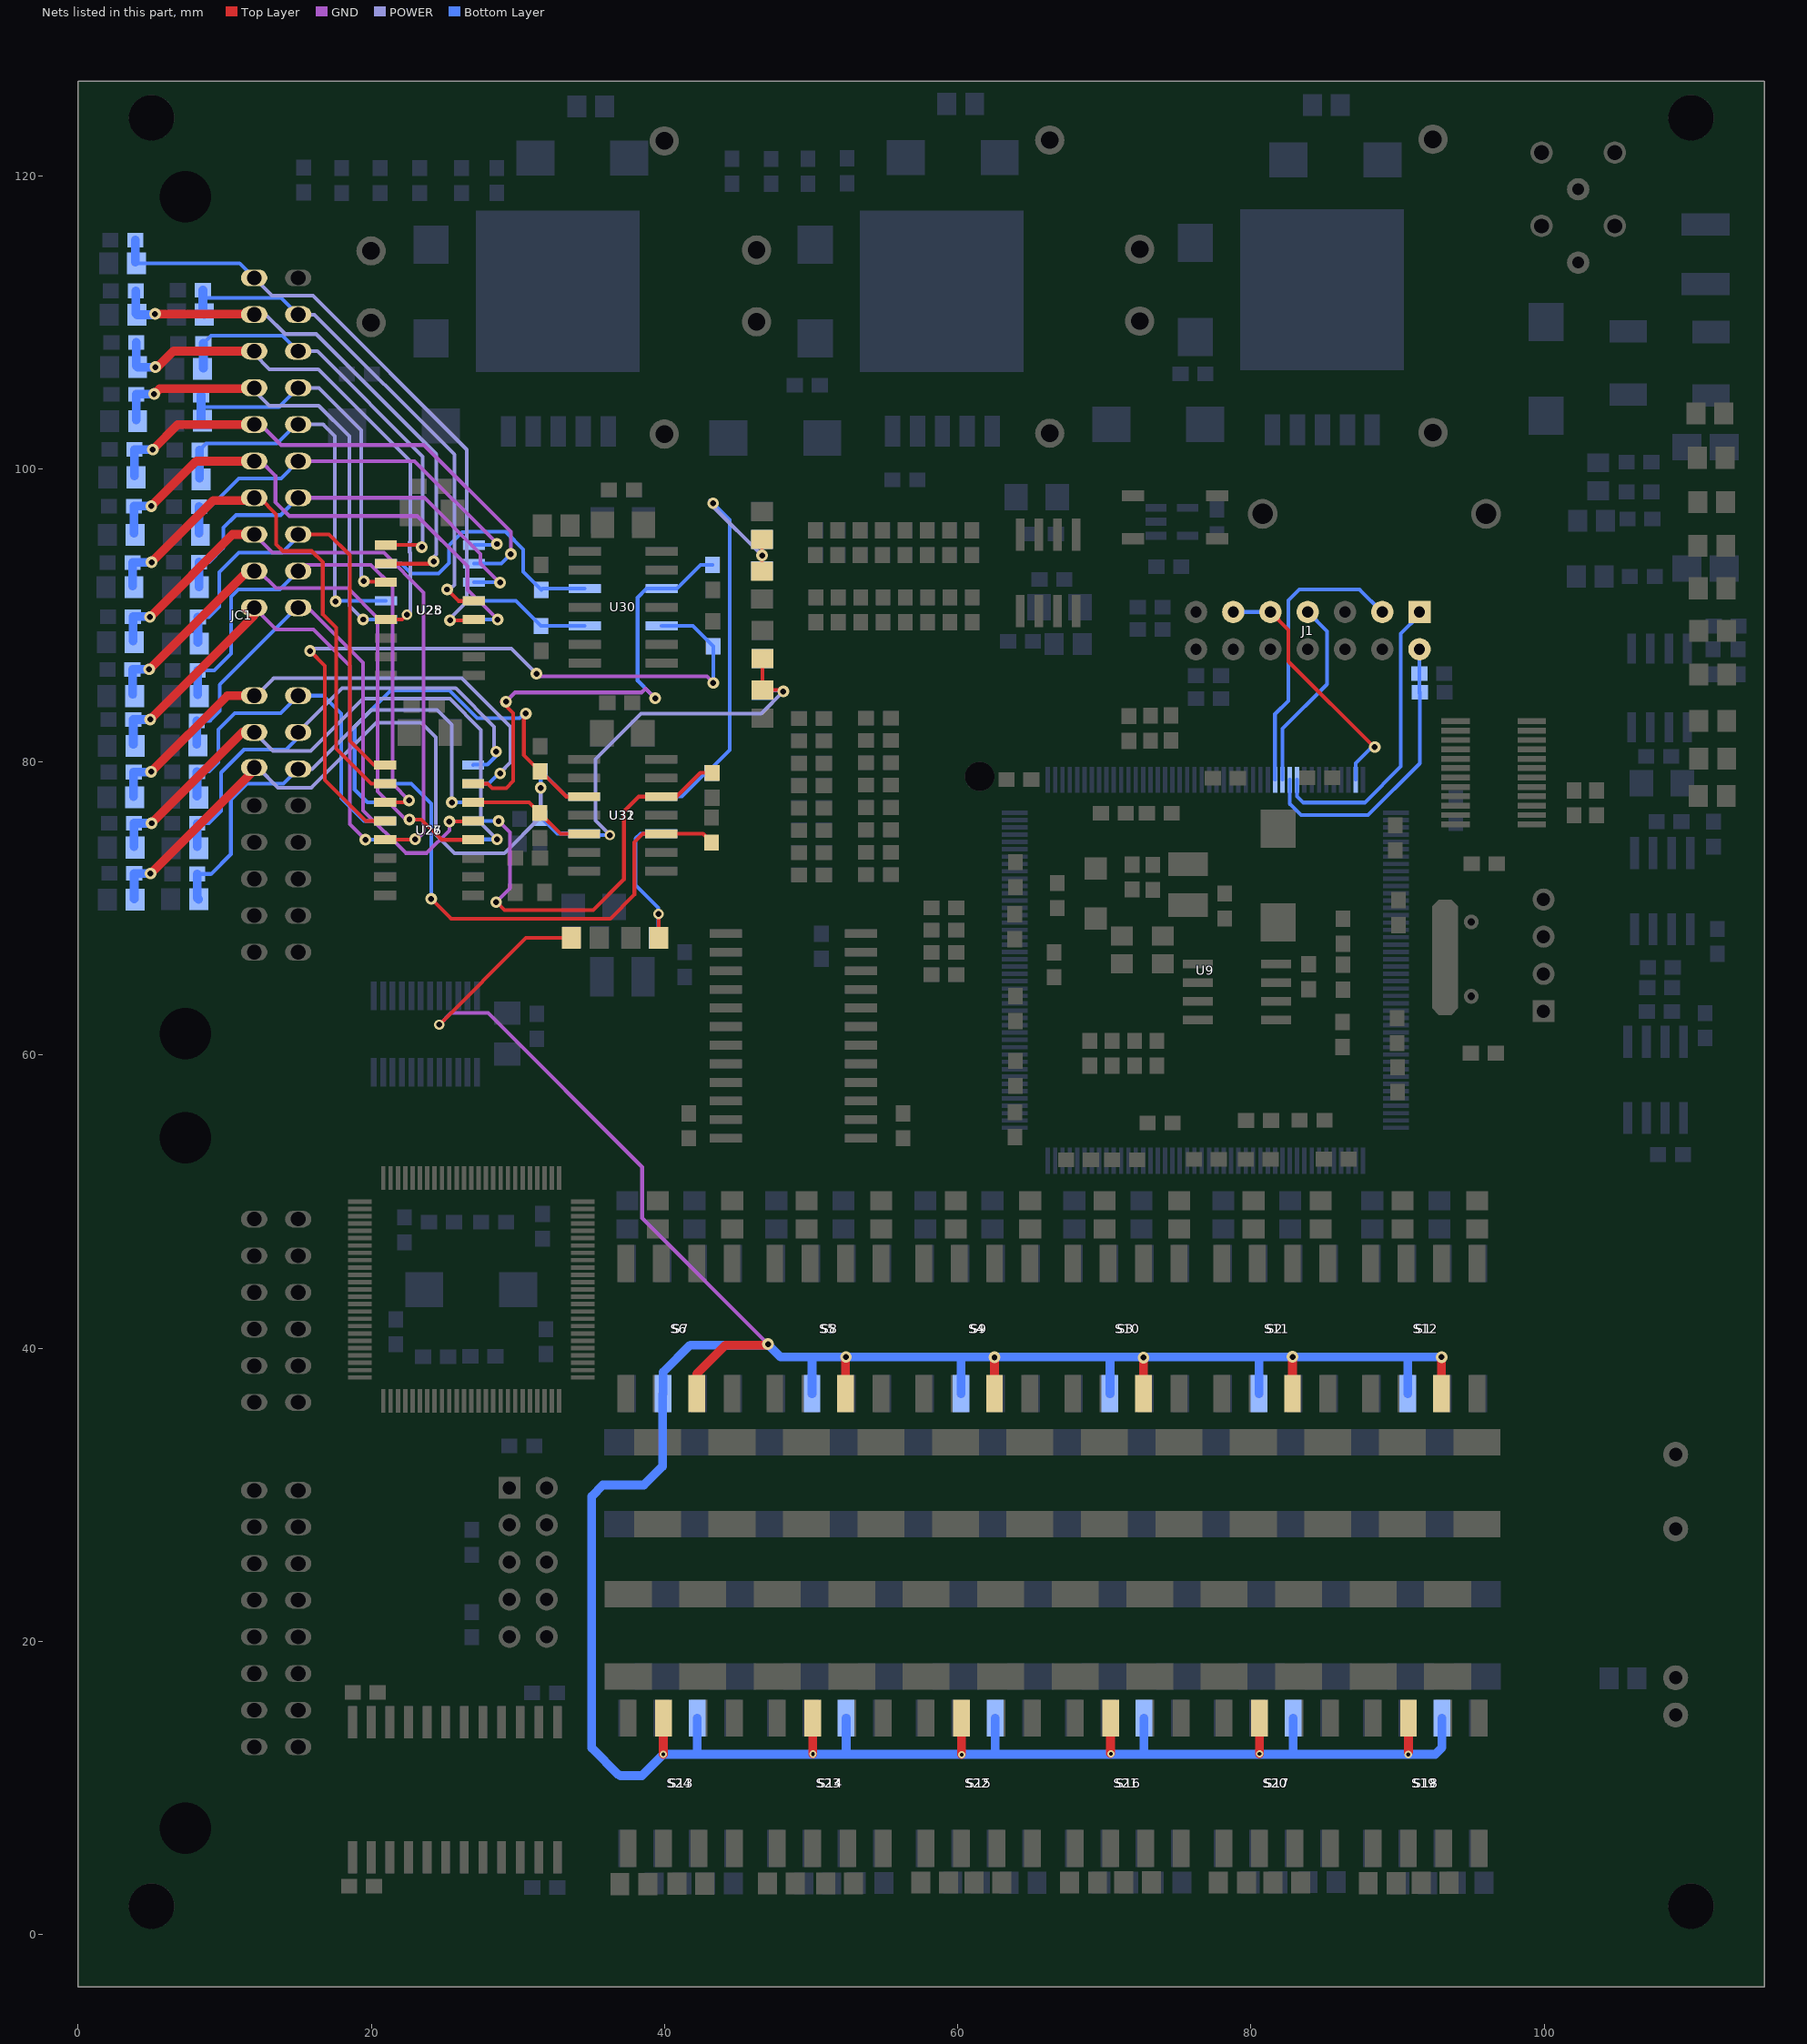
[diagram p0: the nets of this part, all layers, seen from the top]
# Altium PCB MISC86180.PCBDOC (part 9 of 9)
Units mm, origin at the board's own origin, x right, y up, seen from the top; angles counter-clockwise.
Board outline 115 x 130 mm, 4 copper layers (Top Layer, GND, POWER, Bottom Layer); 475 components, 355 nets, 1755 pads, 459 vias.

## Via types
v1: diameter 0.8, hole 0.4, Top Layer to Bottom Layer, 339 vias
v2: diameter 0.7, hole 0.4, Top Layer to Bottom Layer, 83 vias
v3: diameter 0.5, hole 0.254, Top Layer to Bottom Layer, 37 vias

## Nets (pads, with @x,y where several pads share a name; then routed paths per layer and width w, separated by ;. In a path a pad name is that pad's centre, name@x,y a point inside that pad or via, vN(x,y) a via of type N, cw(c..) or ccw(c..) an arc to the next point about the centre after c; other vN are vias at no path point) (continued)
T0910: C157.2 U28.15 U30.5 | length 18.3
  Bottom Layer w0.254: U28.15@20.998,93.527 22.053,93.527 22.717,92.863 24.593,92.863 25.31,93.58 25.31,94.781 26.211,95.681 26.506,95.681 26.522,95.697 29.163,95.697 30.36,94.5 30.36,92.982 C157.2@31.604,91.738 31.697,91.831 U30.5@34.554,91.831
T1112: C160.2 U28.4 U30.3 | length 8.3
  Bottom Layer w0.254: U28.4@26.998,90.987 29.857,90.987 C160.2@31.568,89.276 34.539,89.276 U30.3@34.554,89.291
T1314: C163.2 U27.15 U30.10 | length 33.2
  Top Layer w0.254: U27.15@26.934,78.517 27.943,78.517 28.24,78.22 29.2,78.22 29.68,78.7 29.68,83.34 v1@28.91,84.11
  GND w0.254: v1(29.18,84.11) 29.81,84.74 38.43,84.74 38.7,85.01 v1(39.36,84.35)
  Bottom Layer w0.254: v1@39.21,84.5 39.055,84.655 ; v1(39.36,84.35) 39.055,84.655 ; C163.2@43.252,93.438 42.448,93.438 40.841,91.831 U30.10@39.804,91.831 38.771,91.831 38.16,91.22 38.16,85.55 39.055,84.655
T1516: C166.2 U27.4 U30.12 | length 49.6
  Top Layer w0.254: v1(15.82,87.57) 16.83,86.56 16.83,78.76 19.613,75.977 U27.4@20.934,75.977
  GND w0.254: v1(31.26,86.02) 31.45,85.83 42.88,85.83 v1(43.32,85.39)
  POWER w0.254: v1(15.82,87.57) 15.98,87.73 29.55,87.73 v1(31.26,86.02)
  Bottom Layer w0.254: U30.12@39.804,89.291 41.924,89.291 C166.2@43.318,87.896 43.318,85.392 v1(43.32,85.39)
T1718: C169.2 U27.14 U31.5 | length 8.5
  Top Layer w0.254: U27.14@26.934,77.247 30.751,77.247 C169.2@31.488,76.51 32.903,75.095 U31.5@34.514,75.095
T1920: C172.2 U26.14 U31.3 | length 28.6
  Top Layer w0.254: v1(30.54,83.31) 30.49,83.31 30.4,83.22 30.4,80.472 C172.2@31.512,79.36 31.58,79.36 33.305,77.635 U31.3@34.514,77.635
  Bottom Layer w0.254: U26.14@20.941,77.25 19.73,77.25 18.86,78.119 18.86,82.41 21.33,84.88 25.32,84.88 27.215,82.985 30.115,82.985 30.44,83.31 v1(30.54,83.31)
T2122: C175.2 U26.15 U31.10 | length 34.6
  Top Layer w0.254: v1(24.08,70.66) 25.44,69.3 36.3,69.3 37.94,70.94 37.94,74.51 38.525,75.095 U31.10@39.764,75.095 42.626,75.095 C175.2@43.212,74.51
  Bottom Layer w0.254: U26.15@20.941,78.52 22.72,78.52 24.08,77.16 v1(24.08,70.66)
T2324: C178.2 U26.4 U31.12 | length 29.6
  Top Layer w0.254: v1(28.51,70.44) 28.54,70.44 29.08,69.9 35.14,69.9 37.23,71.99 37.23,76.64 38.225,77.635 U31.12@39.764,77.635 40.825,77.635 42.442,79.252 C178.2@43.248,79.252
  GND w0.254: v1(28.51,70.44) 28.53,70.44 29.46,71.37 29.46,75.19 v1(28.68,75.97)
  Bottom Layer w0.254: U26.4@26.941,75.98 28.67,75.98 v1(28.68,75.97)
T\R\S\T\: C52.2 J1.2 R5.2 U9.78 | length 20.2
  Bottom Layer w0.254: U9.78@82.639,78.793 82.639,77.141 83.41,76.37 87.98,76.37 91.51,79.9 C52.2@91.51,84.762 ; C52.2@91.47,84.702 91.486,84.718 J1.2@91.486,87.693 J1.2@91.54,87.639
TCK: J1.9 J1.11 U9.87 | length 17.6
  Top Layer w0.254: J1.9@81.326,90.233 82.55,89.009 82.55,86.85 88.38,81.02 v1(88.43,81.02)
  Bottom Layer w0.254: J1.11@78.786,90.233 J1.9@81.326,90.233 ; U9.87@87.139,78.793 87.139,79.919 88.24,81.02 v1(88.43,81.02)
TDI: J1.3 U9.76 | length 20
  Bottom Layer w0.254: U9.76@81.639,78.793 81.63,78.803 81.63,83.26 82.54,84.17 82.54,91.03 83.29,91.78 87.399,91.78 J1.3@88.946,90.233
TDO: J1.7 U9.77 | length 13.2
  Bottom Layer w0.254: U9.77@82.139,78.793 82.15,78.804 82.15,82.27 85.18,85.3 85.18,88.919 J1.7@83.866,90.233
TEMP1: C100.2 JC1.11 R106.1 U25.12 | length 44
  Top Layer w0.254: JC1.11@12.01,113.022 JC1.11@12.588,113.022 ; v1(25.37,89.67) U25.12@27.18,89.67
  POWER w0.254: JC1.11@12.01,113.022 13.222,111.81 16.02,111.81 26.52,101.31 26.52,90.93 25.34,89.75 25.34,89.7 v1(25.37,89.67)
  Bottom Layer w0.254: R106.1@3.9,114.103 R106.1@3.991,114.012 3.999,114.02 11.012,114.02 JC1.11@12.01,113.022
  Bottom Layer w0.6: R106.1@3.9,114.103 C100.2@3.9,115.598
TEMP2: C101.2 JC1.2 R107.1 U25.13 | length 36.4
  Top Layer w0.254: v1(25.17,91.77) 25.96,90.98 U25.13@27.29,90.98
  POWER w0.254: JC1.2@15.01,110.522 16.108,110.522 25.66,100.97 25.66,92.09 25.34,91.77 v1(25.17,91.77)
  Bottom Layer w0.254: C101.2@8.51,112.188 C101.2@8.601,112.097 ; R107.1@8.601,110.522 8.601,111.67 13.862,111.67 JC1.2@15.01,110.522
  Bottom Layer w0.6: C101.2@8.51,112.188 8.51,110.613 R107.1@8.601,110.522
TEMP3: C102.2 JC1.12 R108.1 U25.2 | length 36.4
  Top Layer w0.254: v1(5.25,110.56) v1@5.288,110.522 ; JC1.12@11.972,110.522 JC1.12@12.01,110.522 JC1.12@12.058,110.522 ; U25.2@20.991,93.53 21,93.52 v1@23.93,93.52
  Top Layer w0.6: v1(5.25,110.56) JC1.12@11.972,110.56
  POWER w0.254: JC1.12@12.01,110.522 12.788,110.522 14.12,109.19 16.25,109.19 24.44,101 24.44,94.15 24.14,93.85 24.14,93.8 v1(24.25,93.69)
  Bottom Layer w0.254: v1@5.2,110.56 v1(5.25,110.56)
  Bottom Layer w0.6: R108.1@3.929,110.601 C102.2@3.929,112.136 ; R108.1@4.02,110.51 v1@5.2,110.51
TEMP4: C103.2 JC1.3 R109.1 U25.1 | length 29.1
  Top Layer w0.254: U25.1@20.991,94.8 21.011,94.82 23.44,94.82 v1@23.56,94.7
  POWER w0.254: JC1.3@15.01,108.022 16.318,108.022 23.5,100.84 v1@23.5,94.72
  Bottom Layer w0.254: R109.1@8.48,106.81 R109.1@8.539,106.869 ; C103.2@8.539,108.566 9.063,109.09 13.942,109.09 JC1.3@15.01,108.022
  Bottom Layer w0.6: R109.1@8.539,106.869 C103.2@8.539,108.566
  other v1: 23.44,94.66
TEMP5: C104.2 JC1.13 R110.1 U25.5 | length 36.3
  Top Layer w0.254: v1(5.272,106.932) v1@5.28,106.94 ; U25.5@20.991,89.72 22.1,89.72 v2(22.42,90.04)
  Top Layer w0.6: v1(5.272,106.932) 5.412,106.932 6.502,108.022 JC1.13@12.01,108.022
  POWER w0.254: JC1.13@12.01,108.022 12.01,107.83 13.05,106.79 16.38,106.79 22.66,100.51 22.66,95.05 22.613,95.003 22.613,94.317 22.66,94.27 22.66,90.03 22.58,89.95 22.51,89.95 v2(22.42,90.04)
  Bottom Layer w0.6: R110.1@3.97,107.023 C104.2@3.97,108.618 ; R110.1@4.061,106.932 v1(5.272,106.932)
TEMP6: C105.2 JC1.4 R111.1 U25.3 | length 28
  Top Layer w0.254: v1@19.32,92.29 20.96,92.29 U25.3@20.991,92.26
  POWER w0.254: JC1.4@15.01,105.522 16.428,105.522 19.31,102.64 19.31,92.3 v1@19.32,92.29
  Bottom Layer w0.254: C105.2@8.39,105.018 8.481,104.927 R111.1@8.481,103.272 ; 8.491,104.22 13.708,104.22 JC1.4@15.01,105.522
  Bottom Layer w0.6: R111.1@8.39,103.363 C105.2@8.39,105.018
  other v1: 19.49,92.33
TEMP7: C106.2 JC1.14 R112.1 U28.12 | length 32.4
  Top Layer w0.254: JC1.14@11.948,105.46 JC1.14@12.01,105.522
  Top Layer w0.6: v1(5.19,105.1) 5.55,105.46 JC1.14@11.948,105.46
  POWER w0.254: JC1.14@12.01,105.522 12.01,105.33 13.03,104.31 16.41,104.31 18.5,102.22 18.5,90.66 v1(19.44,89.72)
  Bottom Layer w0.254: v1@5.178,105.088 v1(5.19,105.1) ; v1(19.44,89.72) 20.995,89.72 U28.12@20.998,89.717
  Bottom Layer w0.6: R112.1@3.97,103.343 C106.2@3.97,105.088 v1@5.178,105.088
TEMP8: C107.2 JC1.5 R113.1 U28.13 | length 27.1
  POWER w0.254: JC1.5@15.01,103.022 16.718,103.022 17.51,102.23 17.51,91.01 v1@17.49,90.99
  Bottom Layer w0.254: R113.1@8.29,99.373 R113.1@8.381,99.282 ; C107.2@8.29,101.278 8.742,101.73 13.57,101.73 14.862,103.022 JC1.5@15.01,103.022 ; v1@17.49,90.99 20.995,90.99 U28.13@20.998,90.987
  Bottom Layer w0.6: R113.1@8.29,99.373 C107.2@8.29,101.278
  other v1: 17.57,90.95
TEMP9: C108.2 JC1.15 R114.1 U28.2 | length 35.6
  Top Layer w0.254: JC1.15@12.01,103.022 JC1.15@12.078,103.022
  Top Layer w0.6: v1(5.09,101.31) 6.802,103.022 JC1.15@12.01,103.022
  GND w0.254: JC1.15@12.01,103.022 12.438,103.022 13.84,101.62 23.59,101.62 29.51,95.7 v1(29.51,94.18)
  Bottom Layer w0.254: v1@5.082,101.318 v1(5.09,101.31) ; U28.2@26.998,93.527 28.857,93.527 v1(29.51,94.18)
  Bottom Layer w0.6: R114.1@3.85,99.513 C108.2@3.85,101.318 v1@5.082,101.318
TEMP10: C109.2 JC1.6 R115.1 U28.1 | length 26.9
  GND w0.254: JC1.6@15.01,100.522 22.948,100.522 v1@28.42,95.05
  POWER w0.254: v1@28.32,94.82 v1@28.32,94.87
  Bottom Layer w0.254: C109.2@8.25,97.418 9.028,97.418 10.96,99.35 13.838,99.35 JC1.6@15.01,100.522 ; U28.1@26.998,94.797 28.247,94.797 v1@28.32,94.87
  Bottom Layer w0.6: R115.1@8.25,95.593 C109.2@8.25,97.418
  other v1: 28.56,94.87
TEMP11: C110.2 JC1.16 R116.1 U28.5 | length 36
  Top Layer w0.6: v1(4.99,97.45) 8.062,100.522 JC1.16@12.01,100.522
  GND w0.254: JC1.16@12.01,100.522 12.468,100.522 13.46,99.53 13.46,97.72 14.4,96.78 23.14,96.78 26.57,93.35 26.57,91.75 v1(28.61,89.71)
  Bottom Layer w0.254: v1@4.982,97.458 v1(4.99,97.45) ; U28.5@26.998,89.717 28.603,89.717 v1(28.61,89.71)
  Bottom Layer w0.6: R116.1@3.81,95.593 C110.2@3.81,97.458 v1@4.982,97.458
TEMP12: C111.2 JC1.7 R117.1 U28.3 | length 29.4
  GND w0.254: JC1.7@15.01,98.022 23.618,98.022 27.45,94.19 27.45,93.53 v1@28.74,92.24
  Bottom Layer w0.254: R117.1@8.25,91.943 R117.1@8.271,91.922 ; C111.2@8.271,93.617 C111.2@8.25,93.638 8.938,93.638 9.91,94.61 9.91,95.982 10.77,96.842 13.83,96.842 JC1.7@15.01,98.022 ; U28.3@26.998,92.257 28.723,92.257 v1@28.74,92.24
  Bottom Layer w0.6: R117.1@8.25,91.943 C111.2@8.25,93.638
  other v1: 28.78,92.24
TEMP13: C112.2 JC1.17 R118.1 U27.2 | length 36.4
  Top Layer w0.254: JC1.17@12.388,98.022 13.52,96.89 13.52,94.85 13.98,94.39 15.92,94.39 16.69,93.62 16.69,90.07 17.6,89.16 17.6,80.91 19.993,78.517 U27.2@20.934,78.517
  Top Layer w0.6: v1(5.01,93.62) 9.23,97.84 11.828,97.84 JC1.17@12.01,98.022
  Bottom Layer w0.254: v1@4.998,93.608 v1(5.01,93.62)
  Bottom Layer w0.6: R118.1@3.72,92.013 C112.2@3.72,93.608 v1@4.998,93.608
TEMP14: C113.2 JC1.8 R119.1 U27.1 | length 32.3
  Top Layer w0.254: JC1.8@15.01,95.522 17.118,95.522 18.53,94.11 18.53,81.45 20.193,79.787 U27.1@20.934,79.787
  Bottom Layer w0.254: R119.1@8.17,88.173 R119.1@8.261,88.082 ; C113.2@8.17,89.888 8.928,89.888 9.64,90.6 9.64,92.95 10.97,94.28 13.91,94.28 15.01,95.38 JC1.8@15.01,95.522
  Bottom Layer w0.6: R119.1@8.17,88.173 C113.2@8.17,89.888
TEMP15: C114.2 JC1.18 R120.1 U27.5 | length 44.7
  Top Layer w0.254: U27.5@20.934,74.707 20.937,74.71 v1@22.99,74.71
  Top Layer w0.6: v1(4.9,89.89) 10.532,95.522 JC1.18@12.01,95.522
  GND w0.254: JC1.18@12.01,95.522 13.252,94.28 20.85,94.28 23.57,91.56 23.57,75.16 23.14,74.73 v1(22.99,74.73)
  Bottom Layer w0.254: C114.2@3.74,89.918 C114.2@3.768,89.89 ; v1@4.872,89.89 v1(4.9,89.89)
  Bottom Layer w0.6: R120.1@3.74,88.263 C114.2@3.74,89.918 v1@4.872,89.918
TEMP16: C115.2 JC1.9 R121.1 U27.3 | length 37.7
  Top Layer w0.254: U27.3@20.934,77.247 22.437,77.247 v1(22.57,77.38)
  GND w0.254: JC1.9@15.01,93.022 15.428,93.44 19.97,93.44 21.44,91.97 21.44,78.51 v1(22.57,77.38)
  Bottom Layer w0.254: R121.1@8.15,84.603 R121.1@8.261,84.492 ; C115.2@8.15,86.25 9.28,86.25 10.43,87.4 10.43,91.27 10.94,91.78 13.768,91.78 JC1.9@15.01,93.022
  Bottom Layer w0.6: R121.1@8.15,84.603 C115.2@8.15,86.25
TEMP17: C116.2 JC1.19 R122.1 U27.12 | length 42.3
  Top Layer w0.254: JC1.19@11.542,93.022 JC1.19@12.01,93.022 ; v1(22.6,76.08) 23.41,76.08 24.8,74.69 26.917,74.69 U27.12@26.934,74.707
  Top Layer w0.6: v1(4.84,86.32) JC1.19@11.542,93.022
  GND w0.254: JC1.19@12.01,93.022 12.328,93.022 13.5,91.85 18.4,91.85 20.43,89.82 20.43,77.99 v1@22.47,75.95
  Bottom Layer w0.254: R122.1@3.71,84.633 R122.1@3.851,84.492 ; v1@4.836,86.316 v1(4.84,86.32)
  Bottom Layer w0.6: R122.1@3.71,84.633 C116.2@3.71,86.316 v1@4.836,86.316
TEMP18: C117.2 JC1.10 R123.1 U27.13 | length 38.9
  Top Layer w0.254: v1(25.32,75.94) 26.897,75.94 U27.13@26.934,75.977
  GND w0.254: JC1.10@15.01,90.522 15.688,90.522 19.44,86.77 19.44,76.69 22.34,73.79 23.79,73.79 25.32,75.32 v1(25.32,75.94)
  Bottom Layer w0.254: R123.1@8.1,81.203 R123.1@8.181,81.122 ; C117.2@8.1,82.812 8.992,82.812 9.66,83.48 9.66,85.27 14.912,90.522 JC1.10@15.01,90.522 JC1.10@14.99,90.502
  Bottom Layer w0.6: R123.1@8.1,81.203 C117.2@8.1,82.812
TEMP19: C118.2 JC1.20 R124.1 U26.12 | length 35.6
  Top Layer w0.254: JC1.20@11.87,90.382 JC1.20@12.01,90.522
  Top Layer w0.6: v1(4.92,82.9) 12.01,89.99 JC1.20@12.01,90.522
  GND w0.254: JC1.20@12.01,90.522 13.502,89.03 16.05,89.03 18.53,86.55 18.53,75.77 v1(19.6,74.7)
  Bottom Layer w0.254: R124.1@3.77,81.213 R124.1@3.881,81.102 ; v1@4.918,82.898 v1(4.92,82.9) ; v1(19.6,74.7) 20.931,74.7 U26.12@20.941,74.71
  Bottom Layer w0.6: R124.1@3.77,81.213 C118.2@3.77,82.898 v1@4.918,82.898
TEMP20: C119.2 JC1.21 R125.1 U26.13 | length 25
  Bottom Layer w0.254: R125.1@8.11,77.683 R125.1@8.221,77.572 ; C119.2@8.11,79.334 8.126,79.35 8.95,79.35 9.57,79.97 9.57,82.22 10.68,83.33 13.818,83.33 JC1.21@15.01,84.522 16.738,84.522 17.95,83.31 17.95,77.52 19.49,75.98 U26.13@20.941,75.98
  Bottom Layer w0.6: R125.1@8.11,77.683 C119.2@8.11,79.334
TEMP21: C120.2 JC1.29 R126.1 U26.2 | length 37.1
  Top Layer w0.6: v1(4.98,79.33) 10.172,84.522 JC1.29@12.01,84.522
  POWER w0.254: JC1.29@12.01,84.522 12.132,84.522 13.34,85.73 26.17,85.73 29.5,82.4 29.5,79.97 28.79,79.26 v1(28.79,79.22)
  Bottom Layer w0.254: R126.1@3.79,77.653 R126.1@3.861,77.582 ; v1@4.96,79.31 v1(4.98,79.33) ; U26.2@26.941,78.52 28,78.52 28.7,79.22 v1(28.79,79.22)
  Bottom Layer w0.6: R126.1@3.79,77.653 C120.2@3.79,79.31 v1@4.96,79.31
TEMP22: C121.2 JC1.22 R127.1 U26.1 | length 32.7
  POWER w0.254: JC1.22@15.01,82.022 18.018,85.03 25.75,85.03 28.37,82.41 28.37,80.64 28.39,80.62 28.42,80.62 v1(28.51,80.71)
  Bottom Layer w0.254: R127.1@8.119,74.221 R127.1@8.23,74.11 ; C121.2@8.119,75.814 8.904,75.814 9.76,76.67 9.76,79.28 11.31,80.83 11.31,80.84 14.19,80.84 15.01,81.66 JC1.22@15.01,82.022 ; U26.1@26.941,79.79 26.982,79.83 27.92,79.83 28.51,80.42 v1(28.51,80.71)
  Bottom Layer w0.6: R127.1@8.119,74.221 C121.2@8.119,75.814
TEMP23: C122.2 JC1.30 R128.1 U26.5 | length 40.3
  Top Layer w0.254: v1(5.01,75.82) v1@5.14,75.95
  Top Layer w0.6: v1@5.14,75.95 11.212,82.022 JC1.30@12.01,82.022
  POWER w0.254: JC1.30@12.01,82.022 13.282,80.75 15.87,80.75 19.43,84.31 25.35,84.31 27.48,82.18 27.48,75.81 v1(28.57,74.72)
  Bottom Layer w0.254: R128.1@3.82,74.243 R128.1@3.901,74.162 ; v1@5.008,75.822 v1(5.01,75.82) ; U26.5@26.952,74.72 v1(28.57,74.72)
  Bottom Layer w0.6: R128.1@3.82,74.243 C122.2@3.82,75.822 v1@5.008,75.822
TEMP24: C123.2 JC1.23 R129.1 U26.3 | length 33.1
  POWER w0.254: JC1.23@15.01,79.522 15.962,79.522 19.99,83.55 24.48,83.55 25.49,82.54 v1(25.49,77.24)
  Bottom Layer w0.254: C123.2@8.13,72.358 9.058,72.358 10.42,73.72 10.42,77.43 11.512,78.522 14.01,78.522 JC1.23@15.01,79.522 ; v1(25.49,77.24) 25.5,77.25 U26.3@26.941,77.25
  Bottom Layer w0.6: C123.2@8.13,72.358 8.13,70.733 R129.1@8.221,70.642
TEMP25: C124.2 C181.2 JC1.31 R130.1 U32.5 | length 50.4
  Top Layer w0.254: JC1.31@12.01,79.46 JC1.31@12.01,79.622
  Top Layer w0.6: v1(4.94,72.39) JC1.31@12.01,79.46
  POWER w0.254: JC1.31@12.01,79.622 12.258,79.622 13.63,78.25 15.91,78.25 20.33,82.67 23.42,82.67 24.4,81.69 24.4,75.05 25.67,73.78 29.07,73.78 31.55,76.26 v1(31.55,78.23)
  Bottom Layer w0.254: R130.1@3.83,70.672 R130.1@3.885,70.618 ; v1@4.932,72.398 v1(4.94,72.39) ; v1(31.55,78.23) 31.55,79.346 C181.2@31.524,79.372 31.568,79.372 33.295,77.645 U32.5@34.514,77.645
  Bottom Layer w0.6: R130.1@3.83,70.672 C124.2@3.83,72.398 v1@4.932,72.398
TEMPVCU: C127.1 C128.2 C187.2 R133.2 R134.1 U32.10 | length 33.3
  Top Layer w0.254: R134.1@46.65,93.011 v1(46.65,94.09) R133.2@46.65,95.175
  POWER w0.254: v1@43.31,97.43 v1(46.65,94.09)
  Bottom Layer w0.254: U32.10@39.764,77.645 41.185,77.645 42.792,79.252 C187.2@43.212,79.252 ; C187.2@43.212,79.482 C187.2@43.212,79.252 ; v1(43.31,97.65) 43.12,97.84 44.45,96.51 44.45,80.82 43.212,79.582 C187.2@43.212,79.252 ; C128.2@46.65,93.029 v1(46.65,94.09) C127.1@46.65,95.193
TMS: J1.1 U9.79 | length 20.6
  Bottom Layer w0.254: U9.79@83.139,78.793 83.139,77.651 83.56,77.23 87.76,77.23 90.22,79.69 90.22,88.75 91.486,90.016 J1.1@91.486,90.233 J1.1@91.486,90.086
VB: R171.2 R172.1 U32.12 | length 11
  Top Layer w0.254: v2(39.58,69.63) 39.591,69.641 39.595,69.641 39.597,69.639 R171.2@39.597,67.992
  Bottom Layer w0.254: R172.1@39.579,67.992 39.579,70.061 38.03,71.61 38.03,74.78 38.355,75.105 U32.12@39.764,75.105
VCELL: R170.1 S1.7 S2.7 S3.7 S4.7 S5.7 S6.7 S7.7 S8.7 S9.7 S10.7 S11.7 S12.7 S13.7 S14.7 S15.7 S16.7 S17.7 S18.7 S19.7 S20.7 S21.7 S22.7 S23.7 S24.7 | length 249.3
  Top Layer w0.254: v2(24.64,62.08) 30.552,67.992 R170.1@33.633,67.992 ; v3(39.91,12.31) v3@39.937,12.337 ; S13.7@39.937,14.747 S13.7@39.937,14.774 ; v1@47.06,40.21 v1@47.07,40.21 ; S14.7@50.097,14.761 S14.7@50.097,14.774 ; v1@62.503,39.19 v1@62.503,39.39 ; v3@90.737,12.307 v3@90.737,12.45 ; v1@92.983,39.393 v1(92.99,39.4)
  Top Layer w0.6: v3(39.91,12.31) S13.7@39.91,14.747 ; S6.7@42.183,36.902 42.183,38.253 44.14,40.21 v1@47.06,40.21 ; v3(50.11,12.32) S14.7@50.11,14.761 ; S5.7@52.343,36.902 v1@52.343,39.383 ; v3@60.257,12.293 S15.7@60.257,14.774 ; S4.7@62.503,36.902 v1@62.503,39.19 ; v3@70.417,12.363 S16.7@70.417,14.774 ; S3.7@72.663,36.902 v1@72.663,39.367 ; v3(80.577,12.327) S17.7@80.577,14.774 ; S2.7@82.823,36.902 v1@82.823,39.413 ; v3@90.737,12.45 S18.7@90.737,14.774 ; S1.7@92.983,36.902 v1@92.983,39.393
  GND w0.254: v2(24.64,62.08) 25.43,62.87 27.96,62.87 38.47,52.36 38.47,48.88 v1(47.06,40.29)
  Bottom Layer w0.254: 42.223,12.433 42.223,12.54 ; 52.383,12.367 52.383,12.617 ; 62.543,12.337 62.543,12.59 ; 72.703,12.317 72.703,12.5 ; 80.537,39.237 80.537,39.377 ; 82.863,12.377 82.863,12.51 ; 90.63,39.4 90.697,39.333 ; S12.7@90.697,36.902 S12.7@90.72,36.925
  Bottom Layer w0.6: 42.223,12.54 S24.7@42.223,14.774 ; S8.7@50.057,36.902 50.057,39.377 ; 52.383,12.617 S23.7@52.383,14.774 ; S9.7@60.217,36.902 60.217,39.387 ; 62.543,12.59 S22.7@62.543,14.774 ; S10.7@70.377,36.902 70.377,39.247 ; 72.703,12.5 S21.7@72.703,14.774 ; S11.7@80.537,36.902 80.537,39.237 ; 82.863,12.51 S20.7@82.863,14.774 ; S12.7@90.697,36.902 90.697,39.333 ; v1(92.99,39.4) 90.63,39.4 47.91,39.4 47.09,40.22 41.75,40.22 39.897,38.367 S7.7@39.897,36.902 39.856,36.861 39.856,31.936 38.59,30.67 35.79,30.67 35.03,29.91 35.03,12.74 36.88,10.89 36.94,10.89 36.98,10.85 38.45,10.85 v3(39.91,12.31) 57.39,12.31 92.57,12.31 93.023,12.763 S19.7@93.023,14.774
  other v1: 72.66,39.37 52.37,39.41 62.5,39.39 82.83,39.42
  other v3: 60.27,12.28 90.72,12.29 70.44,12.34
VTREF: C125.1 C126.2 C184.2 R131.2 R132.1 U32.3 | length 32.8
  Top Layer w0.254: R132.1@46.686,87.065 R131.2@46.686,84.901 v1@48.009,84.901
  POWER w0.254: v2(36.27,75.01) 35.28,76 35.28,80.19 38.4,83.31 46.6,83.31 v1(48.1,84.81)
  Bottom Layer w0.254: C184.2@31.488,76.5 31.488,76.322 32.69,75.12 34.498,75.12 U32.3@34.514,75.105 34.608,75.01 v2(36.27,75.01) ; C126.2@46.686,87.047 C125.1@46.686,84.883 v1@48.027,84.883
pads on no net: J3.6 J3.7 J3.8 JC1.0 JC2.0 JC2.20 SW1.3 SW1.4 U4.6 U5.8 U6.5 U6.6 U7.5 U7.6 U8.4 U9.1 U9.2 U9.16 U9.25 U9.26 U9.27 U9.28 U9.64 U9.65 U9.66 U9.67 U9.68 U9.69 U9.72 U9.73 U9.74 U9.75 U9.81 U9.82 U9.88 U9.89 U9.90 U9.91 U9.94 U9.95 U9.100 U9.110 U9.111 U9.112 U9.113 U9.114 U9.115 U9.116 U9.119 U9.122 U9.123 U9.124 U9.127 U9.128 U9.129 U9.130 U9.131 U9.132 U9.133 U9.134 U9.135 U9.136 U9.137 U9.138 U9.141 U9.145 U9.148 U9.149 U9.150 U9.151 U9.152 U9.153 U9.156 U9.157 U9.158 U9.161 U9.162 U9.163 U9.164 U9.165 U9.168 U9.175 U9.176 U10.2 U10.3 U10.6 U10.7 U10.10 U10.11 U10.14 U10.15 U10.16 U10.17 U10.18 U10.19 U10.20 U10.21 U10.22 U10.23 U13.5 U15.6 U16.6 U19.17 U19.18 U19.19 U19.20 U19.21 U19.26 U19.27 U19.28 U19.29 U19.30 U19.33 U19.34 U19.35 U19.36 U19.37 U19.38 U19.39 U19.40 U19.41 U19.42 U19.43 U19.44 U19.47 U19.48 U19.49 U19.77 U19.78 U19.83 U19.84 U19.85 U19.86 U19.87 U19.90 U19.91 U19.92 U19.95 U19.96 U19.98 U19.99 U19.100 U20.18 U20.19 U21.3 U21.4 U21.20 U21.21 U23.3 U23.4 U23.20 U23.21 U24.3 U24.4 U24.20 U24.21 U25.7 U26.7 U27.7 U28.7 U34.1 U34.3 U34.5 U34.7 U34.8
copper on no net:
  other v1: 99.75,103.38 100.81,103.38

## Polygon pours and split planes (outlines as drawn)
GNDA on GND "Top Layer-No Net" (solid, remove dead copper, pour order 1000): -2.19,127.72 -2.19,-2.81 -2,-3 -1.76,-3.24 7.03,-3.24 117.43,-3.24 117.61,-3.06 117.61,-0.56 117.61,127.54 116.75,128.4 116.39,128.76 -1.3,128.76 -1.3,128.62 -2.2,127.72
GNDD on POWER "Top Layer-No Net" (solid, remove dead copper, pour order 1001): -4.39,128.09 -4.39,-1.6 -3.17,-2.82 -2.68,-3.31 9.9,-3.31 118.22,-3.31 118.46,-3.55 120.17,-1.84 120.17,127.6 120.17,127.97 118.86,129.28 118.28,128.7 -3.23,128.7 -3.78,128.7 -4.36,128.12

## Keep-outs
Keep-Out Layer:
  lines w0.3: 0.01,0.36 0.01,127.22 ; 0.01,0.38 ccw(c0.735,0.425) 0.78,-0.3 ; 0.01,127.23 cw(c0.735,127.275) 0.69,128 ; 0.74,128.01 114.29,128.01 ; 0.81,-0.3 114.28,-0.3 ; 114.24,128 cw(c114.285,127.275) 115.01,127.32 ; 114.33,-0.3 ccw(c114.285,0.425) 115.01,0.47 ; 115.01,0.53 115.01,127.27

## Silkscreen, mask and mechanical layers (free items; w line width, h text height)
Top Overlay:
  drawing of 463 lines, arcs and shapes, not listed